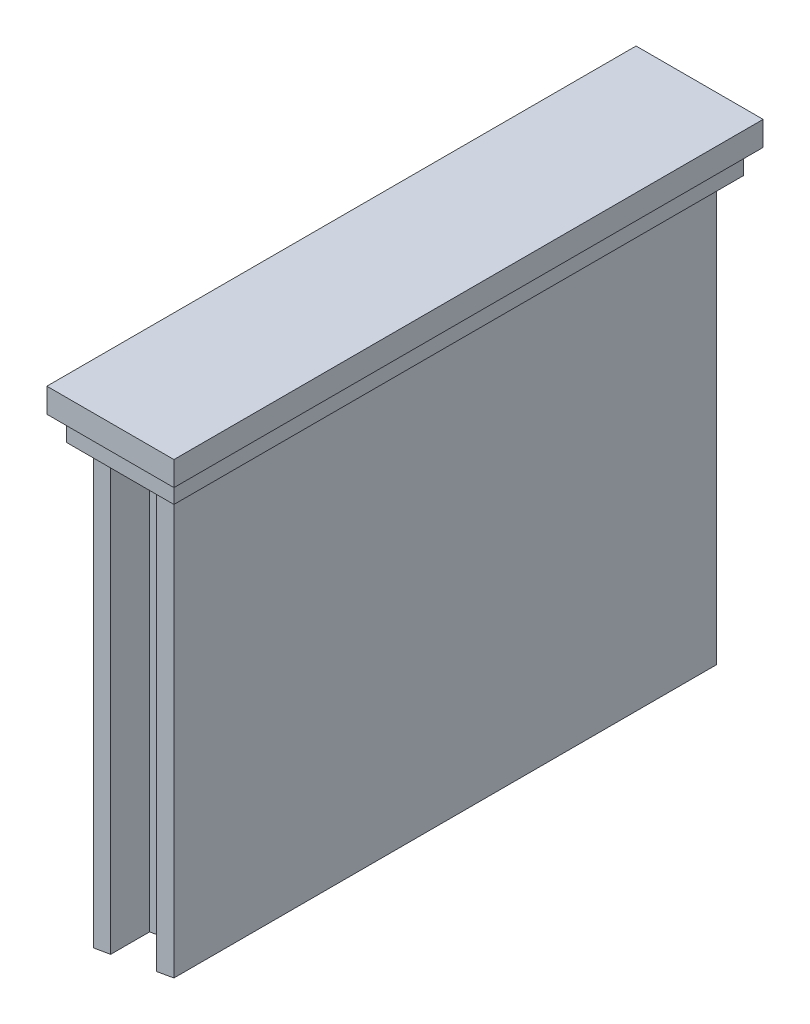
SolidWorks part; units mm, degrees
ref_plane "Front Plane" through (0, 0, 0) normal (0, 0, 1) x (1, 0, 0)
ref_plane "Top Plane" through (0, 0, 0) normal (0, 1, 0) x (1, 0, 0)
ref_plane "Right Plane" through (0, 0, 0) normal (1, 0, 0) x (0, 0, -1)
sketch "Sketch1" plane through (0, 0, 0) normal (0, 1, 0) x (1, 0, 0)
  line L0 (0, 0) -> (26.6288, 0) construction
  line L1 (0, 0) -> (0, 14.5038) construction
  line L2 (-4.14, 27.89) -> (-4.14, -27.89)
  line L3 (-4.14, -27.89) -> (-2.36, -27.89)
  line L4 (-2.36, -27.89) -> (-2.36, -23.89)
  line L5 (-2.36, -23.89) -> (-1.36, -23.89)
  line L6 (-1.36, -23.89) -> (-1.36, -20.89)
  line L7 (-1.36, -20.89) -> (1.36, -20.89)
  line L8 (1.36, -20.89) -> (1.36, -23.89)
  line L9 (1.36, -23.89) -> (2.36, -23.89)
  line L10 (2.36, -23.89) -> (2.36, -27.89)
  line L11 (2.36, -27.89) -> (4.14, -27.89)
  line L12 (4.14, -27.89) -> (4.14, 27.89)
  line L13 (4.14, 27.89) -> (2.36, 27.89)
  line L14 (2.36, 27.89) -> (2.36, 23.89)
  line L15 (2.36, 23.89) -> (1.36, 23.89)
  line L16 (1.36, 23.89) -> (1.36, 20.89)
  line L17 (1.36, 20.89) -> (-1.36, 20.89)
  line L18 (-1.36, 20.89) -> (-1.36, 23.89)
  line L19 (-1.36, 23.89) -> (-2.36, 23.89)
  line L40 (-2.36, 23.89) -> (-2.36, 27.89)
  line L41 (-2.36, 27.89) -> (-4.14, 27.89)
extrude "Boss-Extrude1" add sketch "Sketch1" along normal blind 45
sketch "Sketch2" plane through (0, 0, 27.89) normal (0, 0, 1) x (1, 0, 0)
  line L0 (-4.14, 0) -> (4.14, 0)
  line L1 (4.14, 0) -> (4.14, 1.46)
  line L3 (4.14, 45) -> (4.14, 0) construction
  line L4 (4.14, 1.46) -> (-4.14, 0)
  dimension "D1" = 10
extrude "Cut-Extrude1" cut sketch "Sketch2" against normal through all
sketch "Sketch3" plane through (0, 45, 0) normal (0, 1, 0) x (1, 0, 0)
  line L0 (-5.53, 29.28) -> (5.53, 29.28)
  line L5 (5.53, 29.28) -> (5.53, -29.28)
  line L6 (-5.53, -29.28) -> (5.53, -29.28)
  line L7 (-5.53, 29.28) -> (-5.53, -29.28)
extrude "Boss-Extrude2" add sketch "Sketch3" along normal blind 2.5
sketch "Sketch4" plane through (0, 47.5, 0) normal (0, 1, 0) x (1, 0, 0)
  line L5 (-6.53, 30.28) -> (6.53, 30.28)
  line L6 (6.53, 30.28) -> (6.53, -30.28)
  line L7 (6.53, -30.28) -> (-6.53, -30.28)
  line L8 (-6.53, -30.28) -> (-6.53, 30.28)
extrude "Boss-Extrude3" add sketch "Sketch4" along normal blind 2.5
